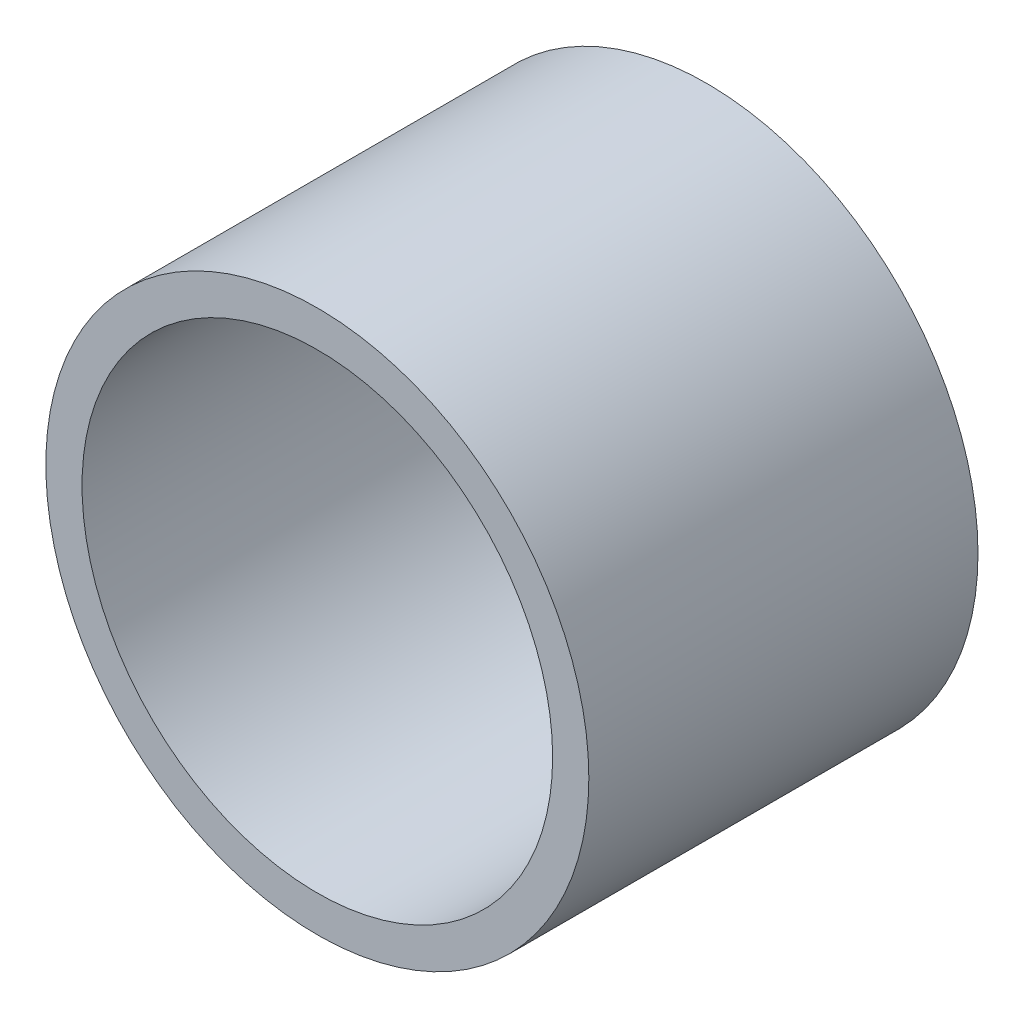
SolidWorks part; units mm, degrees
material "AISI 1045 钢，冷拔"
ref_plane "Front Plane" through (0, 0, 0) normal (0, 0, 1) x (1, 0, 0)
ref_plane "Top Plane" through (0, 0, 0) normal (0, 1, 0) x (1, 0, 0)
ref_plane "Right Plane" through (0, 0, 0) normal (1, 0, 0) x (0, 0, -1)
sketch "Sketch1" plane through (0, 0, 0) normal (0, 0, 1) x (1, 0, 0)
  circle A0 centre (0, 0) radius 13
  circle A1 centre (0, 0) radius 15
  dimension "D1" = 26
  dimension "D2" = 30
extrude "Boss-Extrude1" add sketch "Sketch1" along normal blind 21.5
